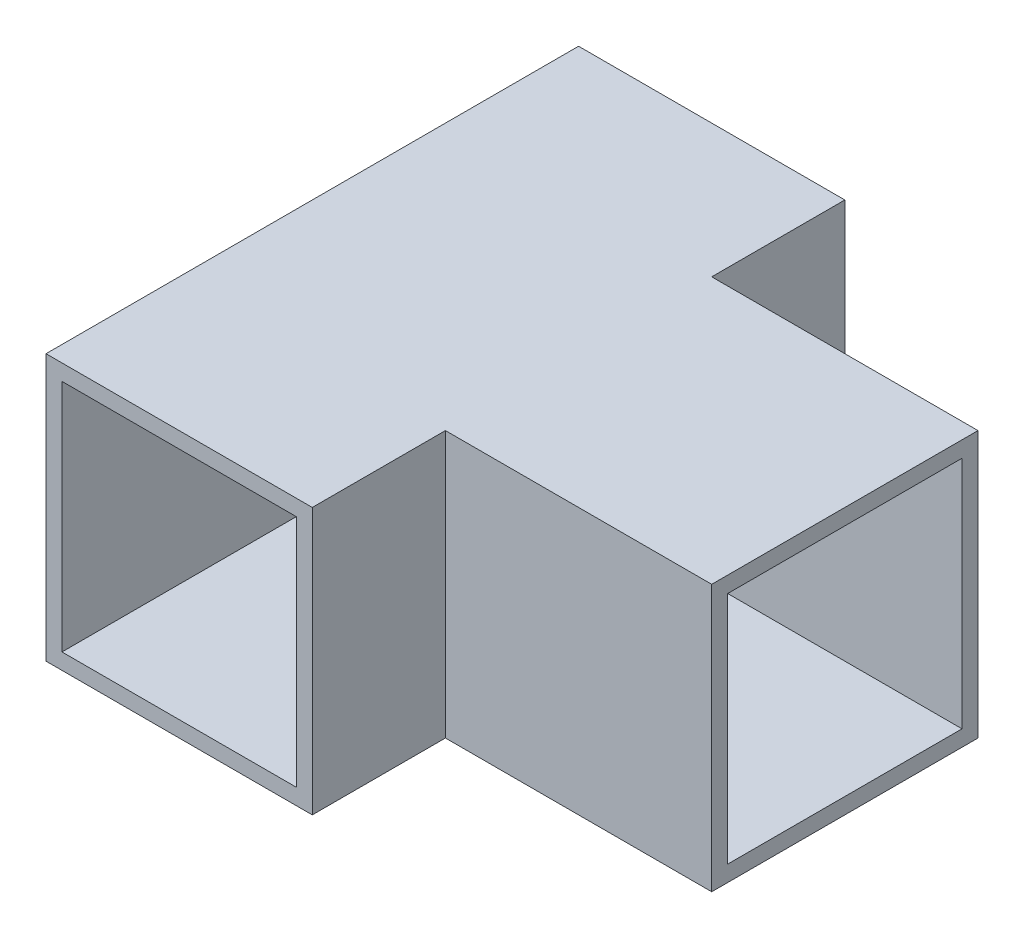
from build123d import *

# Parameters (mm, degrees)
SKETCH_1_W          = 50
SKETCH_1_H          = 50
SKETCH_1_W_2        = 44
SKETCH_1_H_2        = 44
EXTRUDE_1_DEPTH     = 200
SKETCH_2_W          = 56
SKETCH_2_H          = 56
CUT_EXTRUDE_1_DEPTH = 100
EXTRUDE_3_DEPTH     = 100
SKETCH_4_W          = 44
SKETCH_4_H          = 44
CUT_EXTRUDE_2_DEPTH = 100


with BuildPart() as part:
    # 草图1 → 凸台-拉伸1 (new body)
    with BuildSketch(Plane.XY):
        with Locations((25, 25)):
            Rectangle(SKETCH_1_W, SKETCH_1_H)
        with Locations((25, 25)):
            Rectangle(SKETCH_1_W_2, SKETCH_1_H_2, mode=Mode.SUBTRACT)
    extrude(amount=EXTRUDE_1_DEPTH)

    # 草图2 → 切除-拉伸1 (cut)
    with BuildSketch(Plane.XY.offset(200)):
        with Locations((25, 25)):
            Rectangle(SKETCH_2_W, SKETCH_2_H)
    extrude(amount=-CUT_EXTRUDE_1_DEPTH, mode=Mode.SUBTRACT)

    # 草图3 → 凸台-拉伸3 (add)
    with BuildSketch(Plane.ZY):
        Polygon((50, 50), (25, 50), (25, 0), (75, 0), (75, 50), align=None)
        Polygon((50, 47), (28, 47), (28, 3), (72, 3), (72, 47), align=None, mode=Mode.SUBTRACT)
    extrude(amount=-EXTRUDE_3_DEPTH)

    # 草图4 → 切除-拉伸2 (cut)
    with BuildSketch(Plane(origin=(0, 0, 0), x_dir=(-1, 0, 0), z_dir=(0, 0, -1))):
        with Locations((-25, 25)):
            Rectangle(SKETCH_4_W, SKETCH_4_H)
    extrude(amount=-CUT_EXTRUDE_2_DEPTH, mode=Mode.SUBTRACT)


solid = part.part
